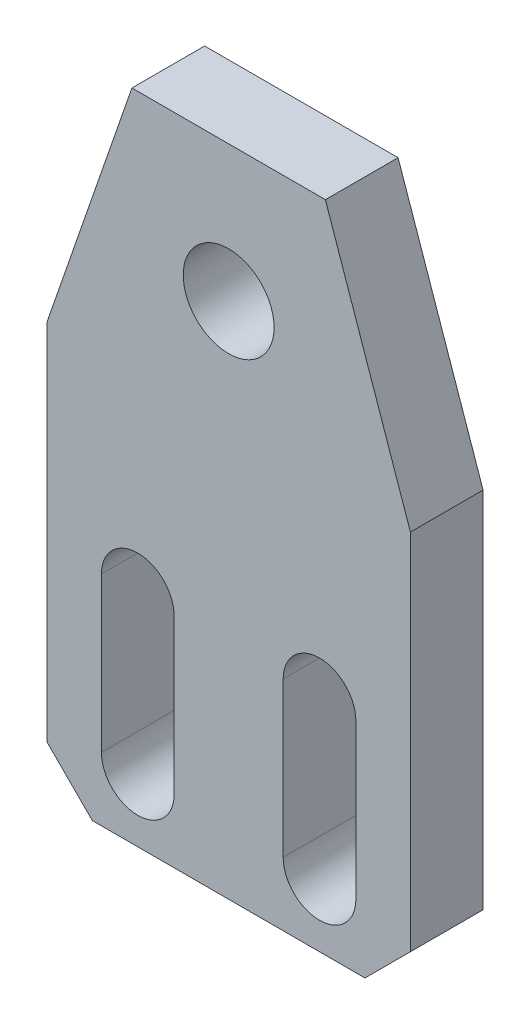
from build123d import *

# Parameters (mm, degrees)
EXTRUDE_1_DEPTH = 8
CHAMFER_1_SIZE  = 5


with BuildPart() as part:
    # 草图1 → 凸台-拉伸1 (new body)
    # profile 1 of 2: a face of its own
    with BuildSketch(Plane.XY):
        with BuildLine():
            Line((-20, 45), (-20, 0))
            Line((-20, 0), (0, 0))
            Line((0, 0), (0, 52))
            ThreePointArc((0, 52), (-5, 57), (0, 62))
            Line((0, 62), (0, 72))
            Line((0, 72), (-10.64516129, 72))
            Line((-10.64516129, 72), (-20, 45))
        make_face()
        with BuildLine():
            ThreePointArc((-6, 7), (-10, 3), (-14, 7))
            Line((-14, 7), (-14, 24))
            ThreePointArc((-14, 24), (-10, 28), (-6, 24))
            Line((-6, 24), (-6, 7))
        make_face(mode=Mode.SUBTRACT)
    # profile 2 of 2: a face of its own
    with BuildSketch(Plane.XY):
        with BuildLine():
            Line((0, 52), (0, 0))
            Line((0, 0), (20, 0))
            Line((20, 0), (20, 45))
            Line((20, 45), (10.64516129, 72))
            Line((10.64516129, 72), (0, 72))
            Line((0, 72), (0, 62))
            ThreePointArc((0, 62), (3.535533906, 60.535533906), (5, 57))
            ThreePointArc((5, 57), (3.535533906, 53.464466094), (0, 52))
        make_face()
        with BuildLine():
            ThreePointArc((14, 7), (10, 3), (6, 7))
            Line((6, 7), (6, 24))
            ThreePointArc((6, 24), (10, 28), (14, 24))
            Line((14, 24), (14, 7))
        make_face(mode=Mode.SUBTRACT)
    extrude(amount=EXTRUDE_1_DEPTH)

    # 倒角1
    chamfer_1_edges = [part.edges().sort_by_distance(p)[0] for p in [
        (-20, 0, 4),
        (20, 0, 4),
    ]]
    chamfer(chamfer_1_edges, length=CHAMFER_1_SIZE)


solid = part.part
